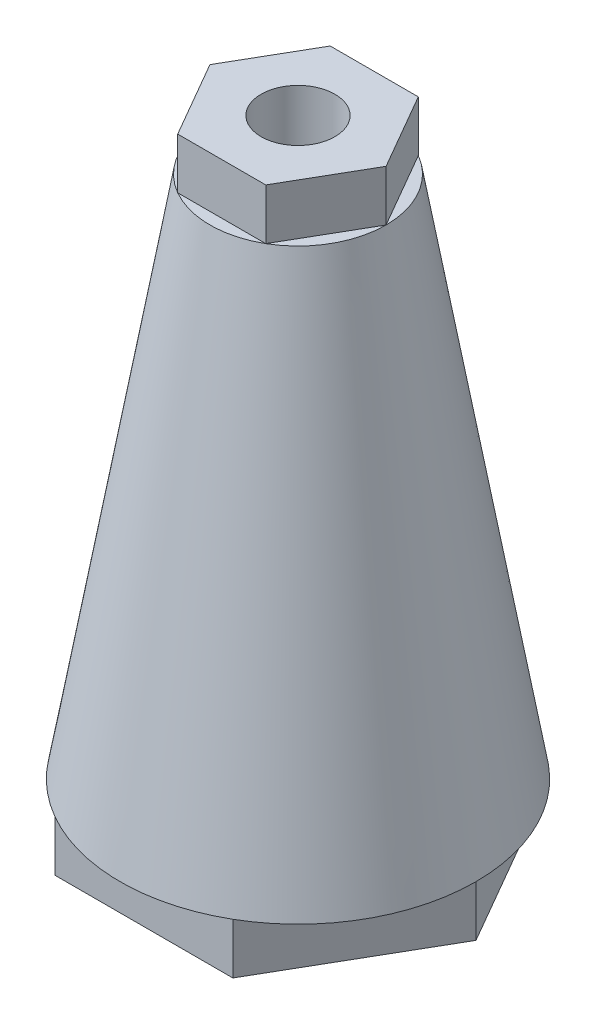
SolidWorks part; units mm, degrees
ref_plane "Front Plane" through (0, 0, 0) normal (0, 0, 1) x (1, 0, 0)
ref_plane "Top Plane" through (0, 0, 0) normal (0, 1, 0) x (1, 0, 0)
ref_plane "Right Plane" through (0, 0, 0) normal (1, 0, 0) x (0, 0, -1)
sketch "Sketch1" plane through (0, 0, 0) normal (0, 1, 0) x (1, 0, 0)
  line L1 (8.6603, -15) -> (17.3205, 0)
  line L2 (17.3205, 0) -> (8.6603, 15)
  line L3 (8.6603, 15) -> (-8.6603, 15)
  line L4 (-8.6603, 15) -> (-17.3205, 0)
  line L5 (-17.3205, 0) -> (-8.6603, -15)
  line L6 (-8.6603, -15) -> (8.6603, -15)
  circle A0 centre (0, 0) radius 15 construction
  dimension "D1" = 30
extrude "Boss-Extrude1" add sketch "Sketch1" along normal blind 10
sketch "Sketch4" plane through (0, 0, 0) normal (0, 0, 1) x (1, 0, 0)
  line L0 (0, 0) -> (17.3205, 0)
  line L1 (17.3205, 0) -> (35, -103)
  line L2 (35, -103) -> (0, -103)
  line L3 (0, -103) -> (0, 0)
  line L4 (-8.6603, 10) -> (8.6603, 10) construction
  dimension "D1" = 113
  dimension "D2" = 35
revolve "Revolve1" add sketch "Sketch4" angle 360 about L3
sketch "Sketch7" plane through (0, -103, 0) normal (0, -1, 0) x (1, 0, 0)
  line L1 (17.5, 30.3109) -> (-17.5, 30.3109)
  line L2 (-17.5, 30.3109) -> (-35, 0)
  line L3 (-35, 0) -> (-17.5, -30.3109)
  line L4 (-17.5, -30.3109) -> (17.5, -30.3109)
  line L5 (17.5, -30.3109) -> (35, 0)
  line L6 (35, 0) -> (17.5, 30.3109)
  circle A0 centre (0, 0) radius 30.3109 construction
  circle A1 centre (0, 0) radius 35 construction
extrude "Boss-Extrude2" add sketch "Sketch7" along normal blind 10
hole_wizard "M16x1.5 Tapped Hole1" positions "Sketch5" profile "Sketch6" tap size "M16x1.5" standard "GB" end condition through all
sketch "Sketch5" plane through (0, 10, 0) normal (0, 1, 0) x (1, 0, 0)
  point P0 (0, 0)
cosmetic thread "Hole Cosmetic Thread1" parameters "D2"=16
sketch "Sketch6" plane through (0, 10, 0) normal (1, 0, 0) x (0, 0, 1)
  line L0 (0, 0) -> (0, 123)
  line L1 (0, 123) -> (7.25, 123)
  line L2 (7.25, 123) -> (7.25, 0)
  line L5 (7.25, 0) -> (0, 0)
  line L11 (0, -6.35) -> (0, 107.95) construction
  dimension "通孔螺纹孔钻头直径" = 14.5
  dimension "通孔螺纹孔钻头深度" = 123
